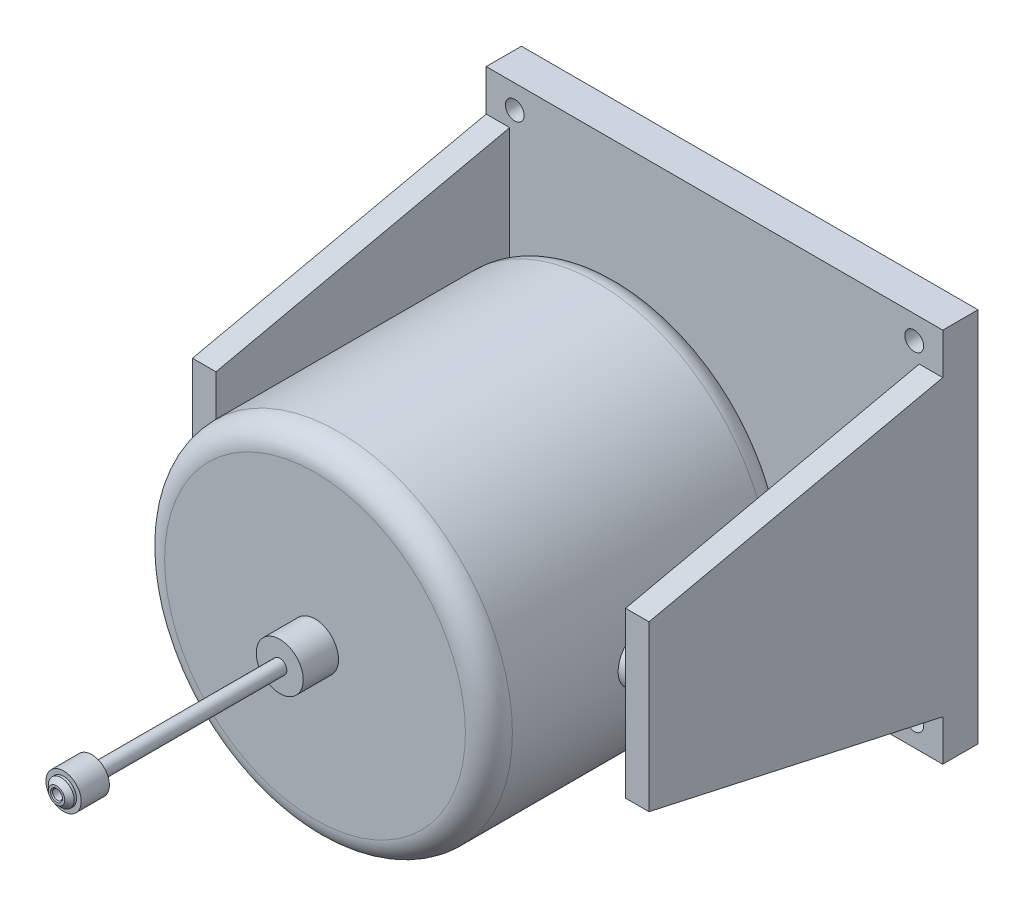
from build123d import *

# Parameters (mm, degrees)
SKETCH1_R                   = 74
BOSS_EXTRUDE1_DEPTH         = 65
FILLET1_R                   = 10
SKETCH2_R                   = 10
BOSS_EXTRUDE2_DEPTH         = 15
BOSS_EXTRUDE3_START         = -200
SKETCH3_W                   = 194.285714286
SKETCH3_H                   = 160
SKETCH3_R                   = 4
BOSS_EXTRUDE3_DEPTH         = 15
BOSS_EXTRUDE4_DEPTH         = 10
SKETCH5_R                   = 10
BOSS_EXTRUDE5_DEPTH         = 90
SKETCH6_R                   = 3
BOSS_EXTRUDE6_DEPTH         = 80
SKETCH7_R                   = 7.5
BOSS_EXTRUDE7_DEPTH         = 12
SKETCH8_R                   = 5.5
BOSS_EXTRUDE8_DEPTH         = 3
CHAMFER1_SIZE               = 2
M5_TAPPED_HOLE1_D           = 4.2
M5_TAPPED_HOLE1_DEPTH       = 14
M5_TAPPED_HOLE1_CSINK_D     = 5.05
M5_TAPPED_HOLE1_CSINK_ANGLE = 90
M5_TAPPED_HOLE1_TIP         = 1.2618073


with BuildPart() as part:
    # Sketch1 → Boss-Extrude1 (new, symmetric)
    with BuildSketch(Plane.XY):
        Circle(SKETCH1_R)
    extrude(amount=BOSS_EXTRUDE1_DEPTH, both=True)

    # Fillet1
    fillet1_edges = [part.edges().sort_by_distance(p)[0] for p in [
        (-74, 0, -65),
        (-74, 0, 65),
    ]]
    fillet(fillet1_edges, radius=FILLET1_R)

    # Sketch2 → Boss-Extrude2 (add)
    with BuildSketch(Plane.XY.offset(65)):
        Circle(SKETCH2_R)
    extrude(amount=BOSS_EXTRUDE2_DEPTH)



with BuildPart() as body_2:
    # Sketch3 → Boss-Extrude3 (new body)
    with BuildSketch(Plane.XY.offset(80).offset(BOSS_EXTRUDE3_START)):
        Rectangle(SKETCH3_W, SKETCH3_H)
        with Locations((-85, 70)):
            Circle(SKETCH3_R, mode=Mode.SUBTRACT)
        with Locations((85, 70)):
            Circle(SKETCH3_R, mode=Mode.SUBTRACT)
        with Locations((85, -70)):
            Circle(SKETCH3_R, mode=Mode.SUBTRACT)
        with Locations((-85, -70)):
            Circle(SKETCH3_R, mode=Mode.SUBTRACT)
    extrude(amount=BOSS_EXTRUDE3_DEPTH)

    # Sketch4 → Boss-Extrude4 (add)
    with BuildSketch(Plane.ZY.offset(97.142857143)):
        Polygon((-105, 62.5), (20, 35), (20, -35), (-105, -62.5), align=None)
    boss_extrude4 = extrude(amount=-BOSS_EXTRUDE4_DEPTH)

    # Mirror1: Boss-Extrude4 across plane
    add(boss_extrude4.mirror(Plane(origin=(0, 0, 0), x_dir=(0, 0, 1), z_dir=(1, 0, 0))))


with BuildPart() as part_1:
    add(part.part)

    add(body_2.part)  # Boss-Extrude5 merges body 2
    # Sketch5 → Boss-Extrude5 (add, symmetric)
    with BuildSketch(Plane(origin=(0, 0, 0), x_dir=(0, 0, -1), z_dir=(1, 0, 0))):
        with Locations(Location((0, 0, 0), (0, 0, 180))):
            Circle(SKETCH5_R)
    extrude(amount=BOSS_EXTRUDE5_DEPTH, both=True)

    # Sketch6 → Boss-Extrude6 (add)
    with BuildSketch(Plane.XY.offset(80)):
        Circle(SKETCH6_R)
    extrude(amount=BOSS_EXTRUDE6_DEPTH)

    # Sketch7 → Boss-Extrude7 (add)
    with BuildSketch(Plane.XY.offset(160)):
        Circle(SKETCH7_R)
    extrude(amount=BOSS_EXTRUDE7_DEPTH)

    # Sketch8 → Boss-Extrude8 (add)
    with BuildSketch(Plane.XY.offset(172)):
        Circle(SKETCH8_R)
    extrude(amount=BOSS_EXTRUDE8_DEPTH)

    # Chamfer1
    chamfer1_edges = [part_1.edges().sort_by_distance(p)[0] for p in [
        (-5.5, 0, 175),
    ]]
    chamfer(chamfer1_edges, length=CHAMFER1_SIZE)

    # M5 Tapped Hole1
    with Locations(Plane.XY.offset(175)):
        with Locations((0, 0)):
            CounterSinkHole(M5_TAPPED_HOLE1_D / 2, M5_TAPPED_HOLE1_CSINK_D / 2, depth=M5_TAPPED_HOLE1_DEPTH, counter_sink_angle=M5_TAPPED_HOLE1_CSINK_ANGLE)
            with Locations((0, 0, -(M5_TAPPED_HOLE1_DEPTH + M5_TAPPED_HOLE1_TIP / 2))):  # 118° drill point
                Cone(0, M5_TAPPED_HOLE1_D / 2, M5_TAPPED_HOLE1_TIP, mode=Mode.SUBTRACT)


solid = part_1.part
